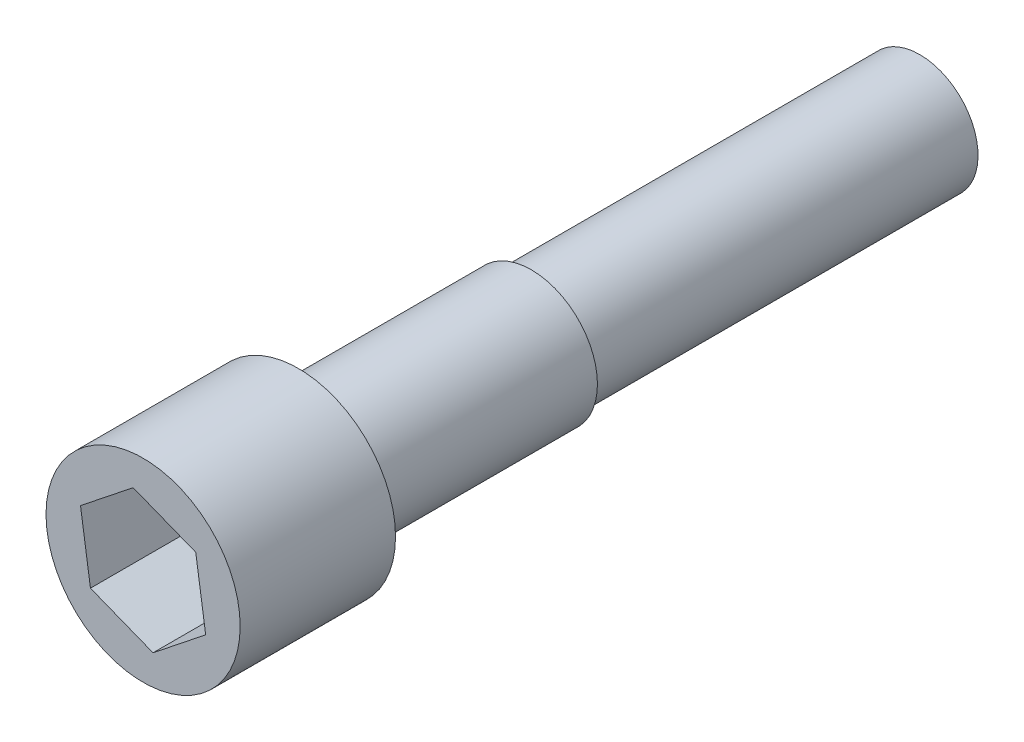
from build123d import *

# Parameters (mm, degrees)
SKETCH_1_R          = 1.7
EXTRUDE_1_DEPTH     = 5.998531593
SKETCH_2_R          = 1.5
EXTRUDE_2_DEPTH     = 10
SKETCH_3_R          = 2.5
EXTRUDE_3_DEPTH     = 4
CUT_EXTRUDE_1_DEPTH = 3


with BuildPart() as part:
    # 草图1 → 凸台-拉伸1 (new body)
    with BuildSketch(Plane.XY):
        with Locations((0, -6)):
            Circle(SKETCH_1_R)
    extrude(amount=-EXTRUDE_1_DEPTH)

    # 草图2 → 凸台-拉伸2 (add)
    with BuildSketch(Plane(origin=(0, 0, -5.998531593), x_dir=(-1, 0, 0), z_dir=(0, 0, -1))):
        with Locations(Location((0, -6, 0), (0, 0, 90))):
            Circle(SKETCH_2_R)
    extrude(amount=EXTRUDE_2_DEPTH)

    # 草图3 → 凸台-拉伸3 (add)
    with BuildSketch(Plane.XY):
        with Locations((0, -6)):
            Circle(SKETCH_3_R)
    extrude(amount=EXTRUDE_3_DEPTH)

    # 草图4 → 切除-拉伸1 (cut)
    with BuildSketch(Plane.XY.offset(4)):
        Polygon((1.355554736, -4.921820351), (-0.255953598, -4.286965337), (-1.611508335, -5.365144986), (-1.355554737, -7.078179649), (0.255953597, -7.713034663), (1.611508334, -6.634855014), align=None)
    extrude(amount=-CUT_EXTRUDE_1_DEPTH, mode=Mode.SUBTRACT)


solid = part.part
